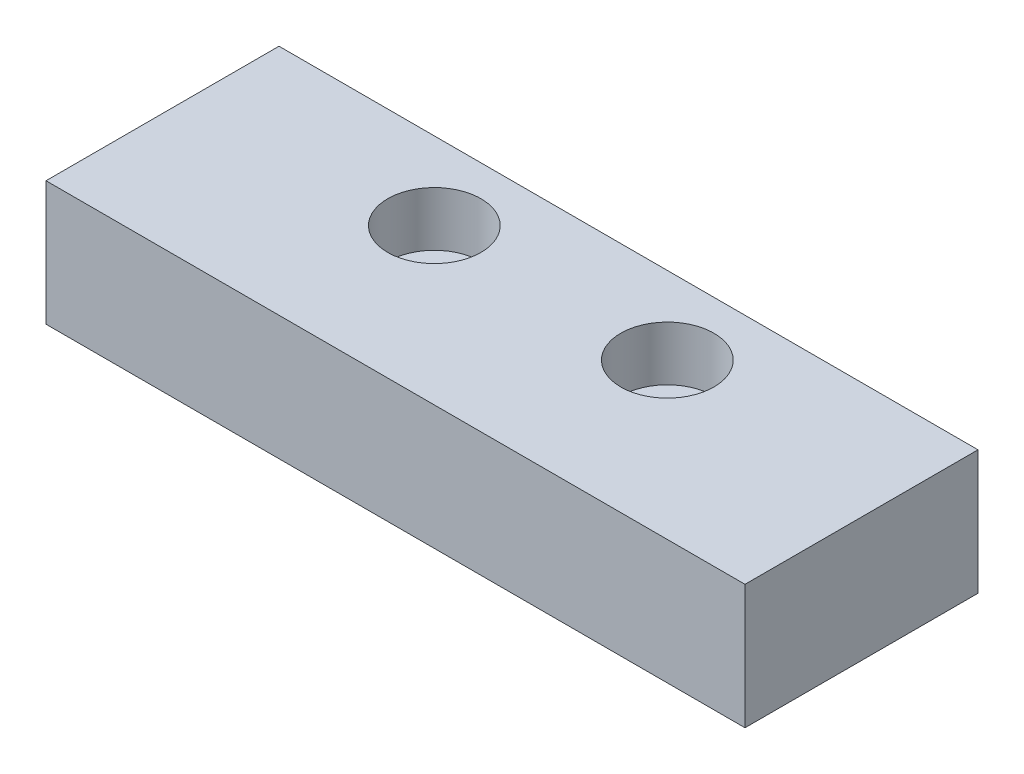
SolidWorks part; units mm, degrees
ref_plane "前视" through (0, 0, 0) normal (0, 0, 1) x (1, 0, 0)
ref_plane "上视" through (0, 0, 0) normal (0, 1, 0) x (1, 0, 0)
ref_plane "右视" through (0, 0, 0) normal (1, 0, 0) x (0, 0, -1)
sketch "草图1" plane through (0, 0, 0) normal (0, 1, 0) x (1, 0, 0)
  line L1 (-22.5, 5) -> (22.5, 5)
  line L2 (-22.5, 5) -> (-22.5, -5)
  line L3 (-22.5, -5) -> (22.5, -5)
  line L4 (22.5, 5) -> (22.5, -5)
  line L5 (-22.5, 5) -> (22.5, -5) construction
  line L6 (-22.5, -5) -> (22.5, 5) construction
  point P0 (0, 0)
  dimension "D1" = 45
  dimension "D2" = 10
extrude "凸台-拉伸1" add sketch "草图1" along normal blind 8
hole_wizard "打孔尺寸(%根据)开槽圆柱头螺钉的类型1" positions "草图3" profile "草图2" counterbore size "M3" standard "GB" end condition through all
sketch "草图3" plane through (0, 8, 0) normal (0, 1, 0) x (1, 0, 0)
  point P0 (-7.5, 0)
  point P2 (7.5, 0)
  dimension "D1" = 7.5
  dimension "D2" = 15
sketch "草图2" plane through (-7.5, 8, 0) normal (1, 0, 0) x (0, 0, 1)
  line L0 (0, 0) -> (0, 8)
  line L1 (0, 8) -> (1.6, 8)
  line L3 (1.6, 8) -> (1.6, 3.5)
  line L4 (1.6, 3.5) -> (3, 3.5)
  line L5 (3, 3.5) -> (3, 0)
  line L7 (3, 0) -> (0, 0)
  line L11 (0, -6.35) -> (0, 107.95) construction
  dimension "通孔孔直径" = 3.2
  dimension "通孔孔深度" = 8
  dimension "柱形沉头孔直径" = 6
  dimension "柱形沉头孔深度" = 3.5
sketch "草图4" plane through (0, 0, 5) normal (0, 0, 1) x (1, 0, 0)
  line L4 (-22.5, 0) -> (22.5, 0)
  line L5 (22.5, 0) -> (22.5, 8)
  line L6 (22.5, 8) -> (-22.5, 8)
  line L7 (-22.5, 8) -> (-22.5, 0)
  line L8 (-22.5, 0) -> (22.5, 0)
  line L9 (22.5, 0) -> (22.5, 8)
  line L10 (22.5, 8) -> (-22.5, 8)
  line L11 (-22.5, 8) -> (-22.5, 0)
  dimension "D1" = 0
extrude "凸台-拉伸2" add sketch "草图4" along normal blind 5
